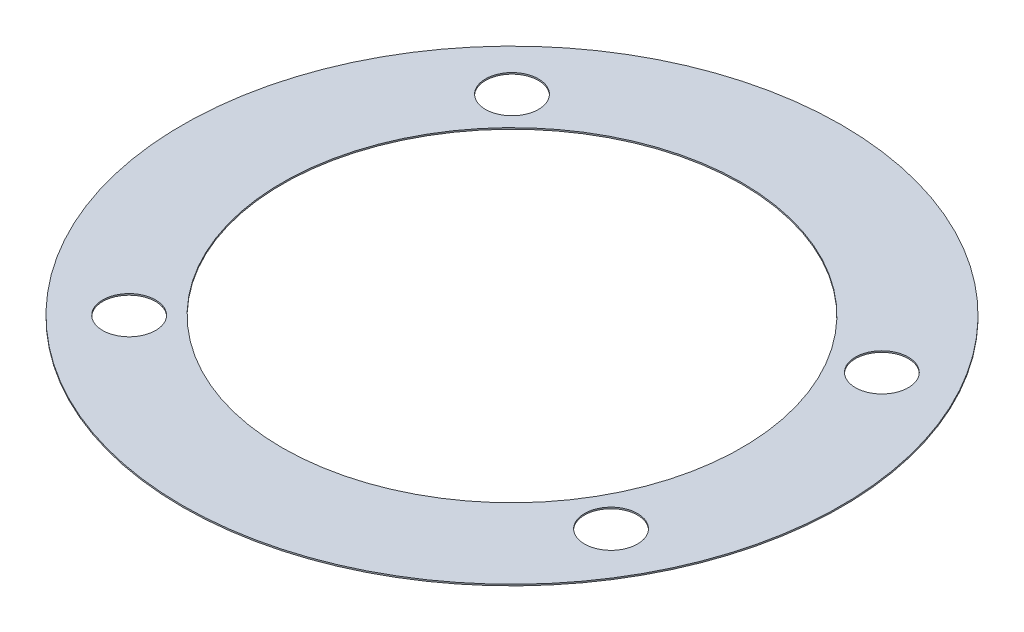
SolidWorks part; units mm, degrees
material "瓦楞纸"
ref_plane "Front Plane" through (0, 0, 0) normal (0, 0, 1) x (1, 0, 0)
ref_plane "Top Plane" through (0, 0, 0) normal (0, 1, 0) x (1, 0, 0)
ref_plane "Right Plane" through (0, 0, 0) normal (1, 0, 0) x (0, 0, -1)
sketch "Sketch1" plane through (0, 0, 0) normal (0, 1, 0) x (1, 0, 0)
  circle A0 centre (0, 0) radius 88.9
  circle A1 centre (0, 0) radius 61.975
  dimension "D1" = 177.8
  dimension "D2" = 123.95
extrude "Boss-Extrude1" add sketch "Sketch1" along normal blind 0.381
hole_wizard "9/16 (0.5625) Diameter Hole1" positions "3DSketch1" profile "Sketch2" hole size "9/16" standard "Ansi Inch"
sketch3d "3DSketch1"
  point P0 (-51.6382, 0.381, -51.64)
  point P2 (63.246, 0.381, 36.53)
  dimension "D1" = 51.64
  dimension "D2" = 36.53
  dimension "D3" = 51.6382
  dimension "D4" = 63.246
sketch "Sketch2" plane through (-51.6382, 0.381, -51.64) normal (1, 0, 0) x (0, 0, 1)
  line L0 (0, 0) -> (0, 20.1724)
  line L1 (0, 20.1724) -> (7.1437, 15.88)
  line L2 (7.1437, 15.88) -> (7.1437, 0)
  line L5 (7.1437, 0) -> (0, 0)
  line L10 (0, 20.1724) -> (-7.1437, 15.88) construction
  line L11 (0, -6.35) -> (0, 107.95) construction
  dimension "孔直径" = 14.2875
  dimension "孔深度" = 15.88
  dimension "导头角度" = 118
mirror "Mirror1" about plane through (0, 0, 0) normal (0, 0, 1) of "9/16 (0.5625) Diameter Hole1"
